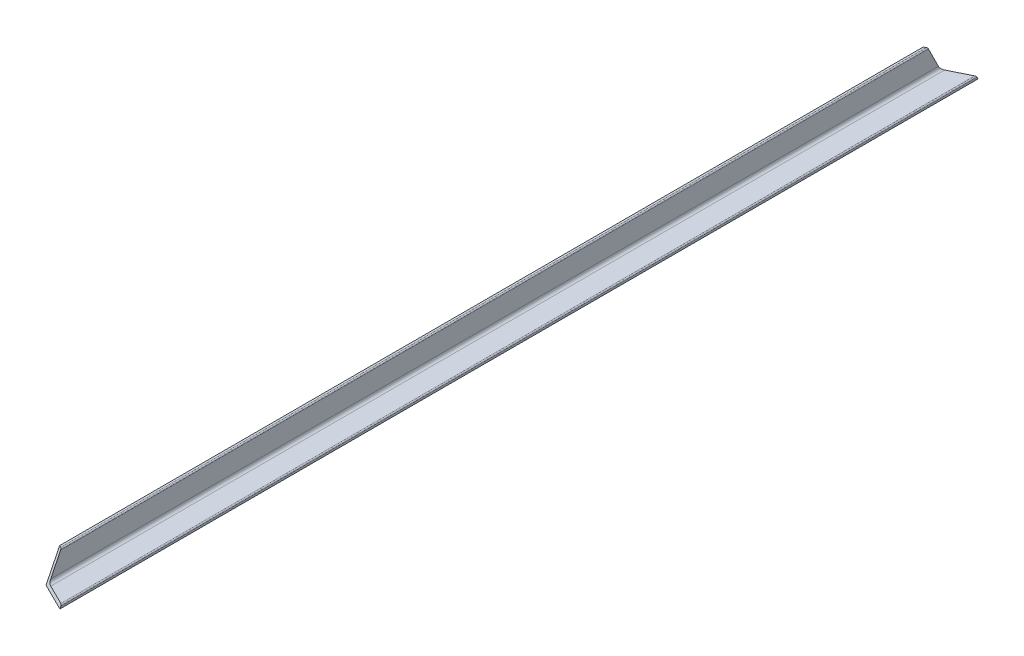
SolidWorks part; units mm, degrees
material "不锈钢角钢70×8/304"
ref_plane "Front Plane" through (0, 0, 0) normal (0, 0, 1) x (1, 0, 0)
ref_plane "Top Plane" through (0, 0, 0) normal (0, 1, 0) x (1, 0, 0)
ref_plane "Right Plane" through (0, 0, 0) normal (1, 0, 0) x (0, 0, -1)
sketch "Sketch1" plane through (0, 0, 0) normal (0, 0, 1) x (1, 0, 0)
  line L0 (0, 70) -> (0, 0)
  line L1 (0, 0) -> (70, 0)
  line L2 (70, 0) -> (70, 5)
  line L3 (67, 8) -> (16, 8)
  line L4 (8, 16) -> (8, 67)
  line L5 (5, 70) -> (0, 70)
  arc A0 (16, 8) -> (8, 16) centre (16, 16) cw
  arc A1 (70, 5) -> (67, 8) centre (67, 5) ccw
  arc A2 (8, 67) -> (5, 70) centre (5, 67) ccw
  dimension "D5" = 8
  dimension "D6" = 3
  dimension "D1" = 70
  dimension "D2" = 70
  dimension "D3" = 8
  dimension "D4" = 8
extrude "Boss-Extrude1" add sketch "Sketch1" along normal blind 2334
ref_plane "Plane1" through (0, 0, 0) normal (0.7071, 0.7071, 0) x (0, 0, -1)
sketch "Sketch3" plane through (0, 0, 0) normal (0.7071, 0.7071, 0) x (0, 0, -1)
  line L0 (0, -49.4975) -> (-69.317, 49.4975)
  line L1 (0, 49.4975) -> (-69.317, 49.4975)
  line L2 (0, 49.4975) -> (0, -49.4975)
  line L3 (-2334, -49.4975) -> (-2334, 49.4975)
  line L4 (-2264.683, 49.4975) -> (-2331, 0) construction
  line L5 (-2264.683, 49.4975) -> (-2334, -49.4975)
  line L7 (-69.317, 49.4975) -> (-3, 0) construction
  line L8 (-2334, 0) -> (0, 0) construction
  line L9 (-3, 0) -> (0, -49.4975) construction
  line L10 (-2334, 49.4975) -> (-2264.683, 49.4975)
  line L12 (-2331, 0) -> (-2334, -49.4975) construction
  dimension "D1" = 35
  dimension "D2" = 35
  dimension "D3" = 3
  dimension "D4" = 3
extrude "Cut-Extrude4" cut sketch "Sketch3" against normal blind 10 and the other way through all
